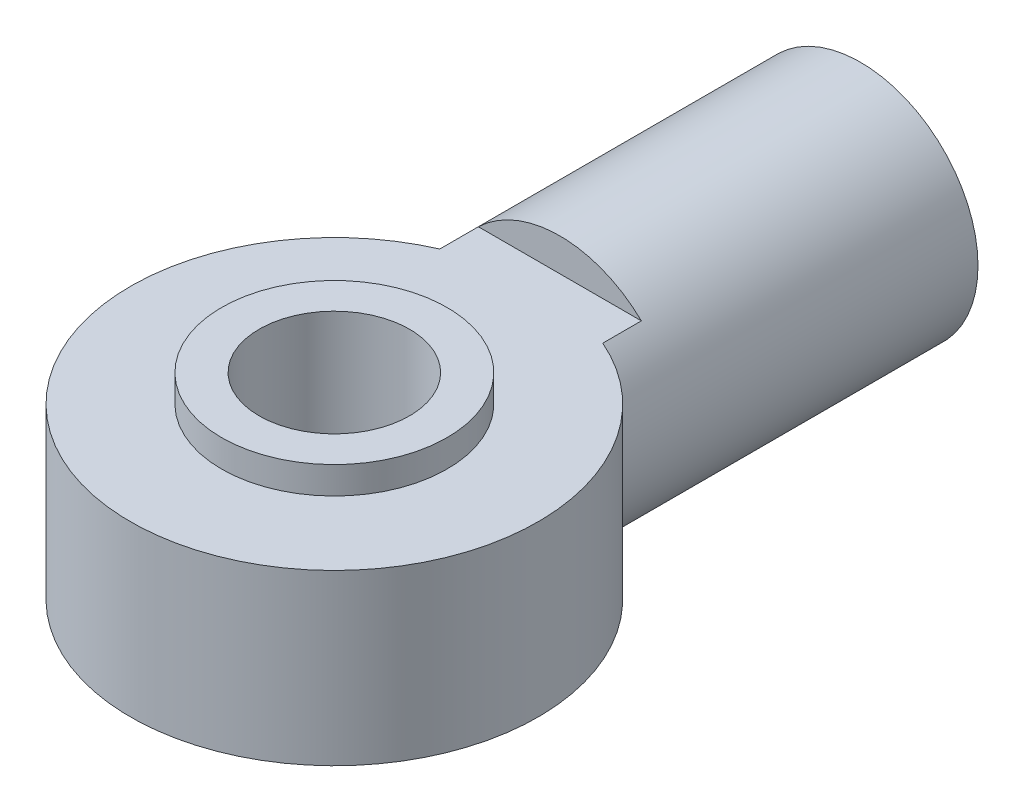
SolidWorks part; units mm, degrees
material "6061 合金"
ref_plane "前视基准面" through (0, 0, 0) normal (0, 0, 1) x (1, 0, 0)
ref_plane "上视基准面" through (0, 0, 0) normal (0, 1, 0) x (1, 0, 0)
ref_plane "右视基准面" through (0, 0, 0) normal (1, 0, 0) x (0, 0, -1)
sketch "草图1" plane through (0, 0, 0) normal (0, 0, 1) x (1, 0, 0)
  circle A0 centre (0, 0) radius 6.25
  dimension "D1" = 12.5
extrude "凸台-拉伸1" add sketch "草图1" along normal blind 28
sketch "草图2" plane through (0, 0, 0) normal (0, 1, 0) x (1, 0, 0)
  line L0 (-6.25, -28) -> (6.25, -28) construction
  circle A0 centre (0, -28) radius 10.85
  dimension "D1" = 21.7
extrude "凸台-拉伸2" add sketch "草图2" along normal mid plane 9
sketch "草图3" plane through (0, 0, 28) normal (0, 0, 1) x (1, 0, 0)
  line L1 (4.3373, -4.5) -> (-4.3373, -4.5)
  line L2 (4.3373, -4.5) -> (-4.3373, -4.5)
  line L3 (-4.3373, 4.5) -> (4.3373, 4.5)
  line L4 (-4.3373, 4.5) -> (4.3373, 4.5)
  arc A1 (-4.3373, -4.5) -> (4.3373, -4.5) centre (0, 0) ccw
  arc A2 (-4.3373, -4.5) -> (4.3373, -4.5) centre (0, 0) ccw
  arc A3 (4.3373, 4.5) -> (-4.3373, 4.5) centre (0, 0) ccw
  arc A4 (4.3373, 4.5) -> (-4.3373, 4.5) centre (0, 0) ccw
  dimension "D1" = 0
  dimension "D2" = 0
extrude "切除-拉伸1" cut sketch "草图3" against normal blind 12
sketch "草图4" plane through (0, -4.5, 0) normal (0, -1, 0) x (1, 0, 0)
  circle A0 centre (0, 28) radius 4
  dimension "D1" = 8
extrude "切除-拉伸2" cut sketch "草图4" against normal through all
hole_wizard "M8 螺纹孔1" positions "草图6" profile "草图7" tap size "M8" standard "GB"
sketch "草图6" plane through (0, 0, 0) normal (0, 0, -1) x (-1, 0, 0)
  point P0 (0, 0)
sketch "草图7" plane through (0, 0, 0) normal (1, 0, 0) x (0, 1, 0)
  line L0 (0, 0) -> (0, 14.0429)
  line L1 (0, 14.0429) -> (3.4, 12)
  line L2 (3.4, 12) -> (3.4, 0)
  line L5 (3.4, 0) -> (0, 0)
  line L10 (0, 14.0429) -> (-3.4, 12) construction
  line L11 (0, -6.35) -> (0, 107.95) construction
  dimension "螺纹孔钻头直径" = 6.8
  dimension "螺纹孔钻头深度" = 12
  dimension "导头角度" = 118
cosmetic thread "孔螺蚊线1" parameters "D1"=12, "D2"=8
sketch "草图8" plane through (0, 0, 0) normal (0, 1, 0) x (1, 0, 0)
  circle A0 centre (0, -28) radius 6
  circle A1 centre (0, -28) radius 4 construction
  circle A2 centre (0, -28) radius 4
  dimension "D1" = 12
extrude "凸台-拉伸3" add sketch "草图8" along normal mid plane 11.9
